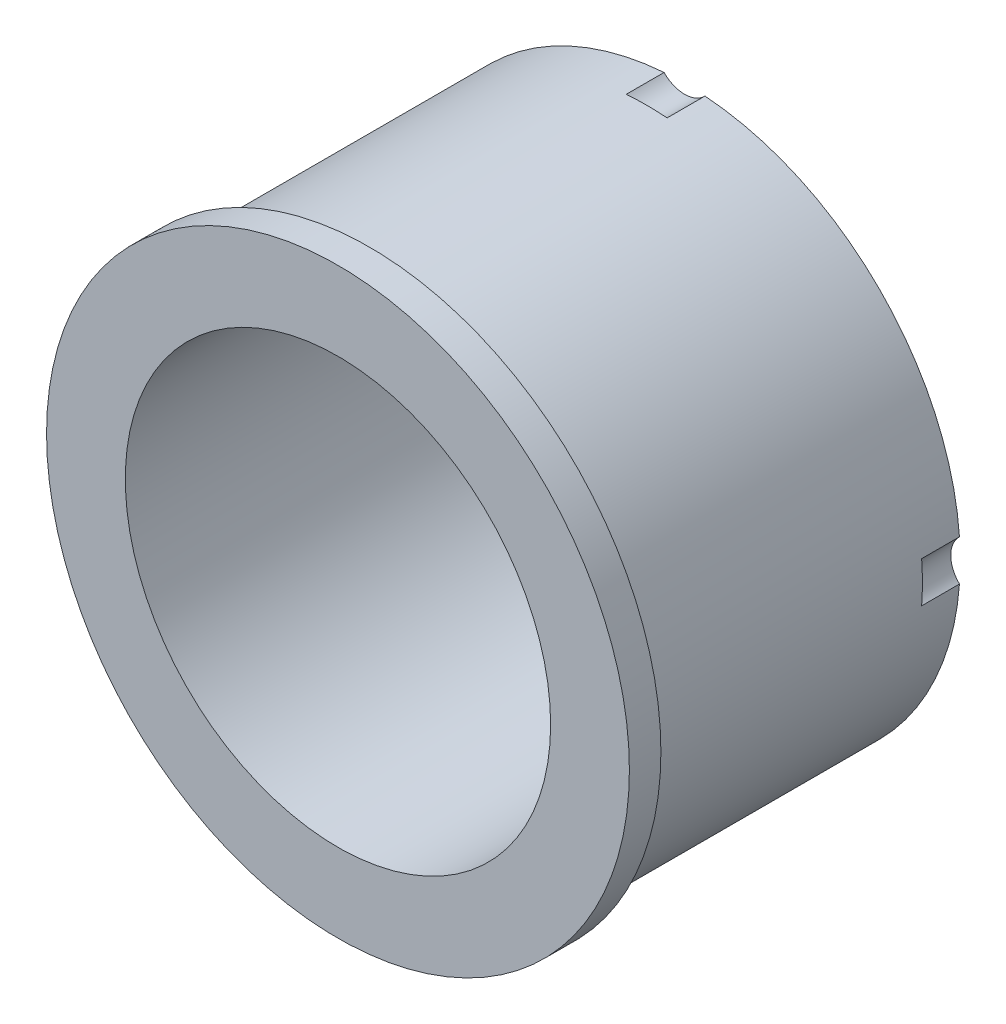
SolidWorks part; units mm, degrees
ref_plane "Front Plane" through (0, 0, 0) normal (0, 0, 1) x (1, 0, 0)
ref_plane "Top Plane" through (0, 0, 0) normal (0, 1, 0) x (1, 0, 0)
ref_plane "Right Plane" through (0, 0, 0) normal (1, 0, 0) x (0, 0, -1)
ref_plane "Plane1" through (0, 234.744, 0) normal (0, 1, 0) x (1, 0, 0)
sketch "Sketch1" plane through (0, 234.744, 0) normal (0, 1, 0) x (1, 0, 0)
  line L0 (613.7306, 1257.693) -> (521.2306, 1257.693)
  line L1 (521.2306, 1257.693) -> (521.2306, 1247.693)
  line L2 (521.2306, 1247.693) -> (613.7306, 1247.693)
  line L3 (613.7306, 1247.693) -> (613.7306, 1257.693)
  line L4 (521.2306, 1257.693) -> (521.2306, 1247.693) construction
  dimension "D1" = 92.5
  dimension "D2" = 10
revolve "Revolve1" add sketch "Sketch1" angle 360 about L4
sketch "Sketch2" plane through (0, 0, -1257.693) normal (0, 0, -1) x (-1, 0, 0)
  circle A0 centre (-521.2306, 234.744) radius 87.5
  dimension "D1" = 175
extrude "Boss-Extrude1" add sketch "Sketch2" along normal blind 100
sketch "Sketch3" plane through (0, 0, -1357.693) normal (0, 0, -1) x (-1, 0, 0)
  arc A0 (-433.9713, 241.2289) -> (-433.9713, 228.259) centre (-427.7306, 234.744) ccw
  arc A1 (-433.9713, 228.259) -> (-433.9713, 241.2289) centre (-521.2306, 234.744) ccw
  circle A2 centre (-521.2306, 234.744) radius 87.5 construction
  dimension "D1" = 9
  dimension "D2" = 87.5
  dimension "D3" = 87.2594
  dimension "D4" = 93.5
  dimension "D5" = 6.4849
extrude "Cut-Extrude1" cut sketch "Sketch3" against normal blind 12
sketch "Sketch4" plane through (0, 0, -1357.693) normal (0, 0, -1) x (-1, 0, 0)
  arc A0 (-514.7457, 147.4846) -> (-527.7156, 147.4846) centre (-521.2306, 141.244) ccw
  arc A1 (-527.7156, 147.4846) -> (-514.7457, 147.4846) centre (-521.2306, 234.744) ccw
  dimension "D1" = 9
  dimension "D2" = 87.5
  dimension "D3" = 80.7744
  dimension "D4" = 87.2594
  dimension "D5" = 6.4849
extrude "Cut-Extrude2" cut sketch "Sketch4" against normal blind 12
sketch "Sketch5" plane through (0, 0, -1357.693) normal (0, 0, -1) x (-1, 0, 0)
  arc A0 (-527.7156, 322.0033) -> (-514.7457, 322.0033) centre (-521.2306, 328.244) ccw
  arc A1 (-514.7457, 322.0033) -> (-527.7156, 322.0033) centre (-521.2306, 234.744) ccw
  dimension "D1" = 9
  dimension "D2" = 87.5
  dimension "D3" = 6.4849
  dimension "D4" = 87.2594
extrude "Cut-Extrude3" cut sketch "Sketch5" against normal blind 12
sketch "Sketch6" plane through (0, 0, -1357.693) normal (0, 0, -1) x (-1, 0, 0)
  arc A0 (-608.49, 228.259) -> (-608.49, 241.2289) centre (-614.7306, 234.744) ccw
  arc A1 (-608.49, 241.2289) -> (-608.49, 228.259) centre (-521.2306, 234.744) ccw
  dimension "D1" = 9
  dimension "D2" = 87.5
  dimension "D3" = 6.4849
  dimension "D4" = 93.7443
  dimension "D5" = 80.7744
extrude "Cut-Extrude4" cut sketch "Sketch6" against normal blind 12
hole_wizard "Hole1" positions "Sketch8" profile "Sketch7" legacy
sketch "Sketch8" plane through (0, 0, -1247.693) normal (0, 0, 1) x (1, 0, 0)
  point P0 (521.2306, 234.744)
sketch "Sketch7" plane through (521.2306, 234.744, -1247.693) normal (1, 0, 0) x (0, -1, 0)
  line L0 (0, 0) -> (0, 110)
  line L1 (0, 110) -> (67.5, 110)
  line L2 (67.5, 110) -> (67.5, 0)
  line L3 (67.5, 0) -> (0, 0)
  line L4 (0, 110) -> (0, -10) construction
  dimension "直径" = 135
  dimension "深度" = 110
